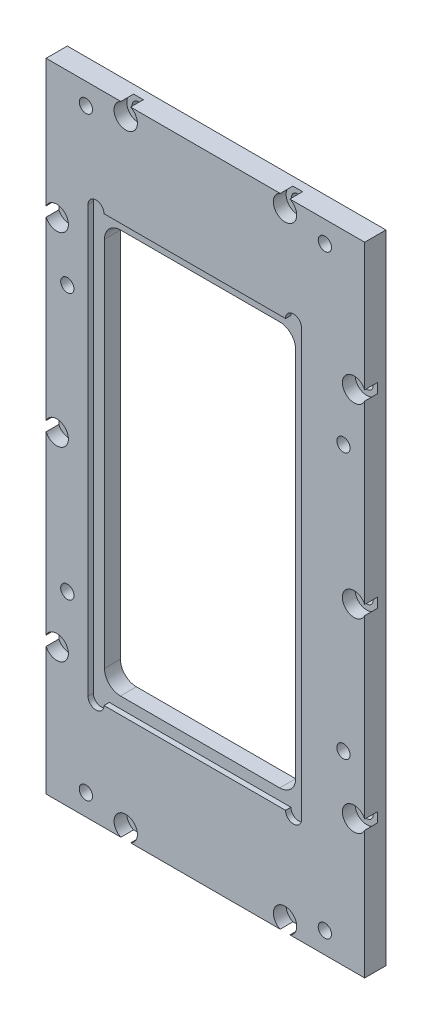
from build123d import *

# Parameters (mm, degrees)
SKETCH_1_W                   = 60
SKETCH_1_H                   = 120
EXTRUDE_1_DEPTH              = 2
SKETCH_2_W                   = 36
SKETCH_2_H                   = 76
CUT_EXTRUDE_1_DEPTH          = 68.201190466
SKETCH_3_W                   = 40.2
SKETCH_3_H                   = 80.2
CUT_EXTRUDE_2_DEPTH          = 1
HOLE_WIZARD_3_0_3_1_D        = 3
HOLE_WIZARD_3_0_3_1_DEPTH    = 1
FILLET_1_R                   = 3
HOLE_WIZARD_M2_1_D           = 2.4
HOLE_WIZARD_M2_1_CBORE_D     = 4.4
HOLE_WIZARD_M2_1_CBORE_DEPTH = 2.4
HOLE_WIZARD_M3_1_D           = 2.5


with BuildPart() as part:
    # 草图1 → 凸台-拉伸1 (new, symmetric)
    with BuildSketch(Plane.XY):
        Rectangle(SKETCH_1_W, SKETCH_1_H)
    extrude(amount=EXTRUDE_1_DEPTH, both=True)

    # 草图2 → 切除-拉伸1 (cut, through all)
    with BuildSketch(Plane.XY.offset(2)):
        with Locations((-2, 0)):
            Rectangle(SKETCH_2_W, SKETCH_2_H)
    extrude(amount=-CUT_EXTRUDE_1_DEPTH, mode=Mode.SUBTRACT)

    # 草图3 → 切除-拉伸2 (cut)
    with BuildSketch(Plane.XY.offset(2)):
        with Locations((-2, 0)):
            Rectangle(SKETCH_3_W, SKETCH_3_H)
    extrude(amount=-CUT_EXTRUDE_2_DEPTH, mode=Mode.SUBTRACT)

    # Ø3.0 (3) 直径孔1
    with Locations(Plane.XY.offset(2)):
        with Locations((-20.6, 40.1), (16.6, 40.1), (16.6, -40.1), (-20.6, -40.1)):
            Hole(HOLE_WIZARD_3_0_3_1_D / 2, depth=HOLE_WIZARD_3_0_3_1_DEPTH)

    # 圆角1
    fillet_1_edges = [part.edges().sort_by_distance(p)[0] for p in [
        (-20, -38, -0.5),
        (-20, 38, -0.5),
        (16, 38, -0.5),
        (16, -38, -0.5),
    ]]
    fillet(fillet_1_edges, radius=FILLET_1_R)

    # M2 六角凹头螺钉的柱形沉头孔1 (through all)
    with Locations(Plane.XY.offset(2)):
        with Locations((-28, 0), (28, 0), (-15, 58), (15, 58), (-28, 35), (28, 35), (-28, -35), (28, -35), (-15, -58), (15, -58)):
            CounterBoreHole(HOLE_WIZARD_M2_1_D / 2, HOLE_WIZARD_M2_1_CBORE_D / 2, HOLE_WIZARD_M2_1_CBORE_DEPTH)

    # M3 螺纹孔1 (through all)
    with Locations(Plane.XY.offset(2)):
        with Locations((-22.5, 56), (22.5, 56), (-26, 25), (26, 25), (26, -25), (-26, -25), (22.5, -56), (-22.5, -56)):
            Hole(HOLE_WIZARD_M3_1_D / 2)


solid = part.part
